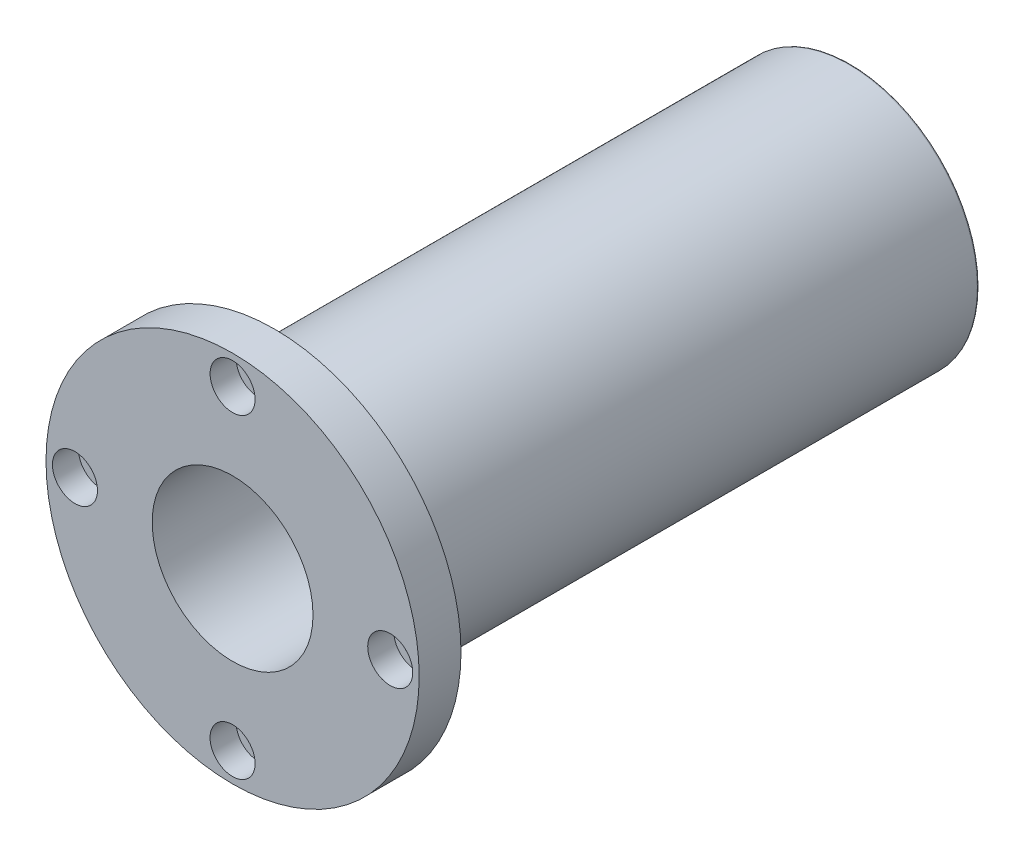
SolidWorks part; units mm, degrees
ref_plane "前视基准面" through (0, 0, 0) normal (0, 0, 1) x (1, 0, 0)
ref_plane "上视基准面" through (0, 0, 0) normal (0, 1, 0) x (1, 0, 0)
ref_plane "右视基准面" through (0, 0, 0) normal (1, 0, 0) x (0, 0, -1)
sketch "草图1" plane through (0, 0, 0) normal (1, 0, 0) x (0, 0, -1)
  line L0 (0, 0) -> (0, 50000) construction
  line L1 (0, 0) -> (50000, 0) construction
  line L3 (0, 40) -> (179, 40)
  line L4 (0, 40) -> (0, 25)
  line L5 (0, 25) -> (179, 25)
  line L6 (179, 40) -> (179, 25)
  dimension "D1" = 179
  dimension "D2" = 80
  dimension "D3" = 50
revolve "旋转1" add sketch "草图1" angle 360 about L1
fillet "圆角1" radius 0.5 1 edges at (40, 0, -179)
sketch "草图2" plane through (0, 0, 0) normal (0, 0, 1) x (1, 0, 0)
  circle A0 centre (0, 0) radius 58
  circle A1 centre (0, 0) radius 25
  dimension "D1" = 116
  dimension "D2" = 50
extrude "凸台-拉伸1" add sketch "草图2" along normal blind 13
sketch "草图3" plane through (0, 0, 0) normal (1, 0, 0) x (0, 0, -1)
  line L0 (0, 0) -> (50000, 0) construction
  line L1 (0, -40) -> (0, 40) construction
  line L2 (-13, 58) -> (-13, -58) construction
  line L4 (-13, 56) -> (-4.9, 56)
  line L5 (-13, 56) -> (-13, 49)
  line L6 (-13, 49) -> (-4.9, 49)
  line L7 (-4.9, 56) -> (-4.9, 49)
  line L8 (0, -58) -> (0, 58) construction
  line L9 (-4.9, 53.5) -> (0, 53.5)
  line L10 (-4.9, 53.5) -> (-4.9, 49)
  line L11 (-4.9, 49) -> (0, 49)
  line L12 (0, 49) -> (50000, 49) construction
  line L13 (0, 53.5) -> (0, 49)
  point P4 (0, 0)
  dimension "D1" = 49
  dimension "D2" = 14
  dimension "D3" = 9
  dimension "D4" = 8.1
revolve "切除-旋转1" cut sketch "草图3" angle 360 about L12
pattern_circular "阵列(圆周)1" count 4 over 360 about axis through (0, 0, 0) along (0, 0, 1) of "切除-旋转1"
